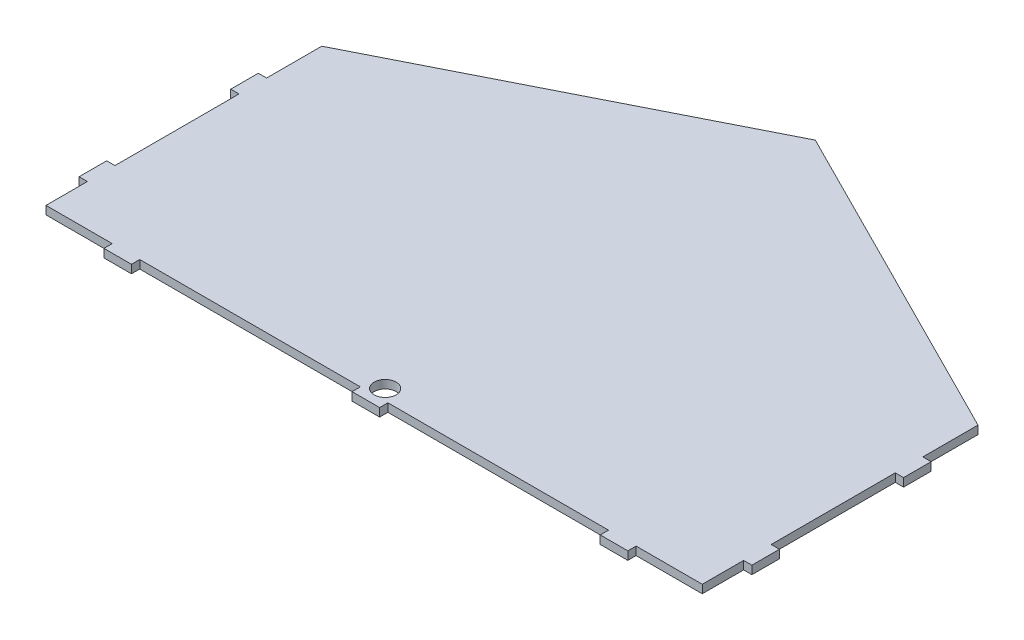
SolidWorks part; units mm, degrees
ref_plane "Front Plane" through (0, 0, 0) normal (0, 0, 1) x (1, 0, 0)
ref_plane "Top Plane" through (0, 0, 0) normal (0, 1, 0) x (1, 0, 0)
ref_plane "Right Plane" through (0, 0, 0) normal (1, 0, 0) x (0, 0, -1)
sketch "Sketch1" plane through (0, 0, 0) normal (0, 1, 0) x (1, 0, 0)
  line L0 (-119, 50) -> (0, 110)
  line L1 (-119, -50) -> (119, -50)
  line L2 (-119, -50) -> (-119, 50)
  line L4 (119, -50) -> (119, 50)
  line L5 (-119, -50) -> (119, 50) construction
  line L6 (-119, 50) -> (119, -50) construction
  line L7 (0, 110) -> (119, 50)
  point P0 (0, 0)
  dimension "D1" = 238
  dimension "D2" = 100
  dimension "D3" = 60
  dimension "D4" = 119
extrude "Boss-Extrude1" add sketch "Sketch1" along normal blind 3
sketch "Sketch3" plane through (0, 3, 0) normal (0, 1, 0) x (1, 0, 0)
  line L0 (119, -50) -> (119, 50) construction
  line L1 (119, 30) -> (122, 30)
  line L2 (119, 30) -> (119, 20)
  line L3 (119, 20) -> (122, 20)
  line L4 (122, 30) -> (122, 20)
  line L5 (0, -1000) -> (0, 49000) construction
  line L6 (119, -35) -> (122, -35)
  line L7 (119, -35) -> (119, -25)
  line L8 (119, -25) -> (122, -25)
  line L9 (122, -35) -> (122, -25)
  line L10 (-119, -50) -> (119, -50) construction
  line L11 (-122, -35) -> (-122, -25)
  line L12 (-119, -25) -> (-122, -25)
  line L13 (-119, -35) -> (-119, -25)
  line L14 (-119, -35) -> (-122, -35)
  line L15 (-122, 30) -> (-122, 20)
  line L16 (-119, 20) -> (-122, 20)
  line L17 (-119, 30) -> (-119, 20)
  line L18 (-119, 30) -> (-122, 30)
  line L19 (-95, -50) -> (-95, -53)
  line L20 (85, -50) -> (95, -50)
  line L21 (85, -50) -> (85, -53)
  line L22 (85, -53) -> (95, -53)
  line L23 (95, -50) -> (95, -53)
  line L24 (-85, -53) -> (-95, -53)
  line L25 (-85, -50) -> (-85, -53)
  line L26 (-85, -50) -> (-95, -50)
  line L28 (-5, -53) -> (5, -53)
  line L29 (-5, -53) -> (-5, -50)
  line L30 (-5, -50) -> (5, -50)
  line L31 (5, -53) -> (5, -50)
  line L32 (-5, -53) -> (5, -50) construction
  line L33 (-5, -50) -> (5, -53) construction
  point P31 (0, -51.5)
  dimension "D1" = 3
  dimension "D2" = 10
  dimension "D3" = 70
  dimension "D4" = 10
  dimension "D5" = 3
  dimension "D6" = 15
  dimension "D7" = 10
  dimension "D8" = 3
  dimension "D9" = 24
  dimension "D10" = 3
  dimension "D11" = 10
extrude "Boss-Extrude2" add sketch "Sketch3" against normal up to surface (3 mm away) up to face at (0, 0, -22)
sketch "Sketch4" plane through (0, 3, 0) normal (0, 1, 0) x (1, 0, 0)
  line L0 (5, -50) -> (85, -50) construction
  circle A0 centre (0, -46) radius 4
  dimension "D1" = 8
  dimension "D2" = 4
extrude "Cut-Extrude1" cut sketch "Sketch4" against normal through all
